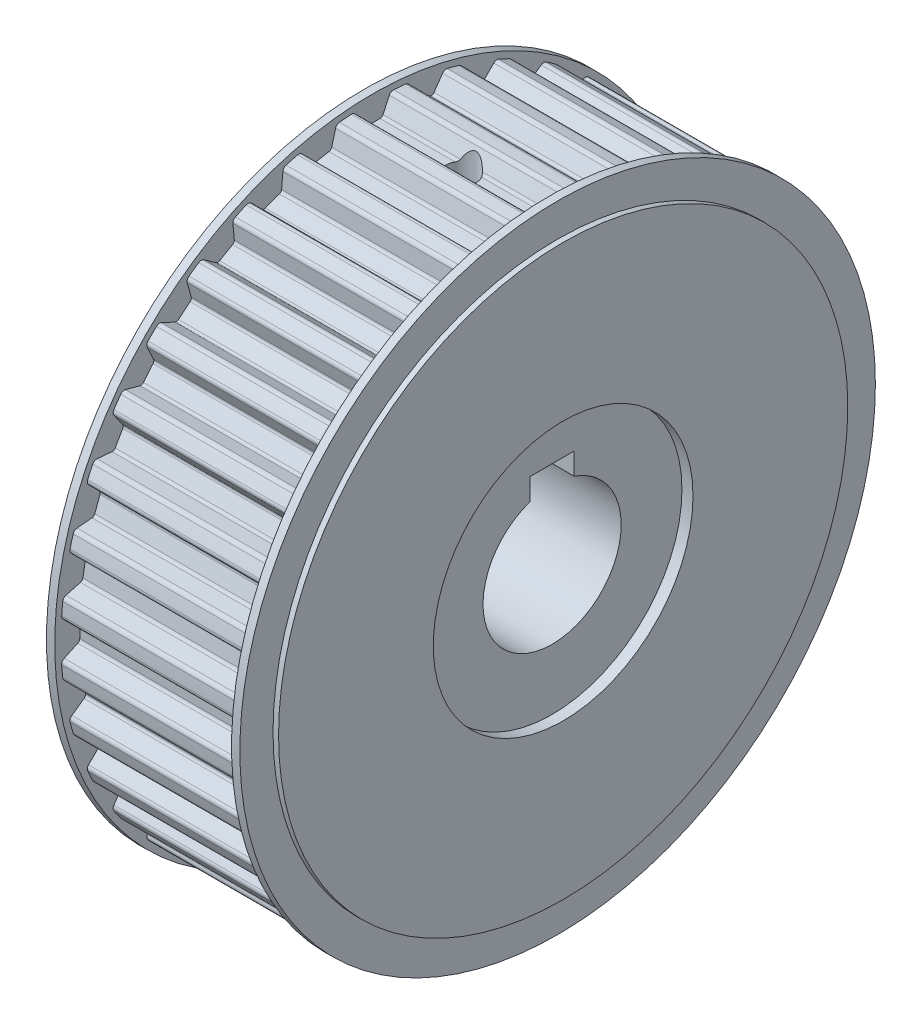
from build123d import *

# Parameters (mm, degrees)
SKETCH_1_R                       = 56.37
EXTRUDE_1_DEPTH                  = 16
CUT_EXTRUDE_2_DEPTH              = 32
FILLET_1_R                       = 0.6
FILLET_2_R                       = 0.8
PATTERN_CIRCULAR_1_COUNT         = 36
FILLET_1_OF_PATTERN_CIRCULAR_1_R = 0.6
FILLET_2_OF_PATTERN_CIRCULAR_1_R = 0.8
SKETCH_6_R                       = 57.5
EXTRUDE_2_DEPTH                  = 1.5
SKETCH_7_R                       = 51.5
EXTRUDE_3_DEPTH                  = 1
SKETCH_8_R                       = 12.5
CUT_EXTRUDE_1_DEPTH              = 90.339241098
SKETCH_11_W                      = 8
SKETCH_11_H                      = 9.02365329
CUT_EXTRUDE_3_DEPTH              = 25
HOLE_WIZARD_M4_1_D               = 3.3
HOLE_WIZARD_M4_1_DEPTH           = 47.1
HOLE_WIZARD_M4_1_TIP             = 0.991420021
SKETCH_14_R                      = 23.5
CUT_EXTRUDE_4_DEPTH              = 2
HOLE_WIZARD_5_5_5_5_1_D          = 5.5
HOLE_WIZARD_5_5_5_5_1_DEPTH      = 35
HOLE_WIZARD_5_5_5_5_1_TIP        = 1.652366702


with BuildPart() as part:
    # 草图1 → 拉伸1 (new, symmetric)
    with BuildSketch(Plane(origin=(0, 0, 0), x_dir=(0, 0, -1), z_dir=(1, 0, 0))):
        Circle(SKETCH_1_R)
    extrude(amount=EXTRUDE_1_DEPTH, both=True)

    # 草图2 → 拉伸2 (cut)
    with BuildSketch(Plane(origin=(16, 0, 0), x_dir=(0, 0, -1), z_dir=(1, 0, 0))):
        with BuildLine():
            Line((-3.285, 56.274200794), (-1.744225866, 52.97))
            Line((-1.744225866, 52.97), (1.744225866, 52.97))
            Line((1.744225866, 52.97), (3.285, 56.274200794))
            ThreePointArc((3.285, 56.274200794), (0, 56.37), (-3.285, 56.274200794))
        make_face()
    cut_extrude_2 = extrude(amount=-CUT_EXTRUDE_2_DEPTH, mode=Mode.SUBTRACT)

    # 圆角1
    fillet_1_edges = [part.edges().sort_by_distance(p)[0] for p in [
        (0, 52.97, -1.744225866),
        (0, 52.97, 1.744225866),
    ]]
    fillet(fillet_1_edges, radius=FILLET_1_R)

    # 圆角2
    fillet_2_edges = [part.edges().sort_by_distance(p)[0] for p in [
        (0, 56.274200794, 3.285),
        (0, 56.274200794, -3.285),
    ]]
    fillet(fillet_2_edges, radius=FILLET_2_R)

    # 阵列(圆周)1: 拉伸2 ×36 about axis
    pattern_circular_1_axis = Axis((0, 0, 0), (1, 0, 0))
    for i in range(1, PATTERN_CIRCULAR_1_COUNT):
        add(cut_extrude_2.rotate(pattern_circular_1_axis, i * 360 / PATTERN_CIRCULAR_1_COUNT), mode=Mode.SUBTRACT)

    # 圆角1 of 阵列(圆周)1
    fillet_1_of_pattern_circular_1_edges = [part.edges().sort_by_distance(p)[0] for p in [
        (0, 52.46814832, 7.480416815),
        (0, 51.862385034, 10.915871127),
        (0, 50.372078504, 16.477770817),
        (0, 49.178957742, 19.755843167),
        (0, 46.745478571, 24.97445609),
        (0, 45.001252706, 27.99554391),
        (0, 41.698540927, 32.712305153),
        (0, 39.456207377, 35.384614217),
        (0, 35.384614217, 39.456207377),
        (0, 32.712305153, 41.698540927),
        (0, 27.99554391, 45.001252706),
        (0, 24.97445609, 46.745478571),
        (0, 19.755843167, 49.178957742),
        (0, 16.477770817, 50.372078504),
        (0, 10.915871127, 51.862385034),
        (0, 7.480416815, 52.46814832),
        (0, 1.744225866, 52.97),
        (0, -1.744225866, 52.97),
        (0, -7.480416815, 52.46814832),
        (0, -10.915871127, 51.862385034),
        (0, -16.477770817, 50.372078504),
        (0, -19.755843167, 49.178957742),
        (0, -24.97445609, 46.745478571),
        (0, -27.99554391, 45.001252706),
        (0, -32.712305153, 41.698540927),
        (0, -35.384614217, 39.456207377),
        (0, -39.456207377, 35.384614217),
        (0, -41.698540927, 32.712305153),
        (0, -45.001252706, 27.99554391),
        (0, -46.745478571, 24.97445609),
        (0, -49.178957742, 19.755843167),
        (0, -50.372078504, 16.477770817),
        (0, -51.862385034, 10.915871127),
        (0, -52.46814832, 7.480416815),
        (0, -52.97, 1.744225866),
        (0, -52.97, -1.744225866),
        (0, -52.46814832, -7.480416815),
        (0, -51.862385034, -10.915871127),
        (0, -50.372078504, -16.477770817),
        (0, -49.178957742, -19.755843167),
        (0, -46.745478571, -24.97445609),
        (0, -45.001252706, -27.99554391),
        (0, -41.698540927, -32.712305153),
        (0, -39.456207377, -35.384614217),
        (0, -35.384614217, -39.456207377),
        (0, -32.712305153, -41.698540927),
        (0, -27.99554391, -45.001252706),
        (0, -24.97445609, -46.745478571),
        (0, -19.755843167, -49.178957742),
        (0, -16.477770817, -50.372078504),
        (0, -10.915871127, -51.862385034),
        (0, -7.480416815, -52.46814832),
        (0, -1.744225866, -52.97),
        (0, 1.744225866, -52.97),
        (0, 7.480416815, -52.46814832),
        (0, 10.915871127, -51.862385034),
        (0, 16.477770817, -50.372078504),
        (0, 19.755843167, -49.178957742),
        (0, 24.97445609, -46.745478571),
        (0, 27.99554391, -45.001252706),
        (0, 32.712305153, -41.698540927),
        (0, 35.384614217, -39.456207377),
        (0, 39.456207377, -35.384614217),
        (0, 41.698540927, -32.712305153),
        (0, 45.001252706, -27.99554391),
        (0, 46.745478571, -24.97445609),
        (0, 49.178957742, -19.755843167),
        (0, 50.372078504, -16.477770817),
        (0, 51.862385034, -10.915871127),
        (0, 52.46814832, -7.480416815),
    ]]
    fillet(fillet_1_of_pattern_circular_1_edges, radius=FILLET_1_OF_PATTERN_CIRCULAR_1_R)

    # 圆角2 of 阵列(圆周)1
    fillet_2_of_pattern_circular_1_edges = [part.edges().sort_by_distance(p)[0] for p in [
        (0, 54.848834973, 13.007005886),
        (0, 55.9897035, 6.536818949),
        (0, 51.756915056, 22.33380048),
        (0, 54.003987398, 16.160019962),
        (0, 47.092387465, 30.981993848),
        (0, 50.377387465, 25.292206946),
        (0, 40.996981511, 38.688815011),
        (0, 45.220096107, 33.65590302),
        (0, 33.65590302, 45.220096107),
        (0, 38.688815011, 40.996981511),
        (0, 25.292206946, 50.377387465),
        (0, 30.981993848, 47.092387465),
        (0, 16.160019962, 54.003987398),
        (0, 22.33380048, 51.756915056),
        (0, 6.536818949, 55.9897035),
        (0, 13.007005886, 54.848834973),
        (0, -3.285, 56.274200794),
        (0, 3.285, 56.274200794),
        (0, -13.007005886, 54.848834973),
        (0, -6.536818949, 55.9897035),
        (0, -22.33380048, 51.756915056),
        (0, -16.160019962, 54.003987398),
        (0, -30.981993848, 47.092387465),
        (0, -25.292206946, 50.377387465),
        (0, -38.688815011, 40.996981511),
        (0, -33.65590302, 45.220096107),
        (0, -45.220096107, 33.65590302),
        (0, -40.996981511, 38.688815011),
        (0, -50.377387465, 25.292206946),
        (0, -47.092387465, 30.981993848),
        (0, -54.003987398, 16.160019962),
        (0, -51.756915056, 22.33380048),
        (0, -55.9897035, 6.536818949),
        (0, -54.848834973, 13.007005886),
        (0, -56.274200794, -3.285),
        (0, -56.274200794, 3.285),
        (0, -54.848834973, -13.007005886),
        (0, -55.9897035, -6.536818949),
        (0, -51.756915056, -22.33380048),
        (0, -54.003987398, -16.160019962),
        (0, -47.092387465, -30.981993848),
        (0, -50.377387465, -25.292206946),
        (0, -40.996981511, -38.688815011),
        (0, -45.220096107, -33.65590302),
        (0, -33.65590302, -45.220096107),
        (0, -38.688815011, -40.996981511),
        (0, -25.292206946, -50.377387465),
        (0, -30.981993848, -47.092387465),
        (0, -16.160019962, -54.003987398),
        (0, -22.33380048, -51.756915056),
        (0, -6.536818949, -55.9897035),
        (0, -13.007005886, -54.848834973),
        (0, 3.285, -56.274200794),
        (0, -3.285, -56.274200794),
        (0, 13.007005886, -54.848834973),
        (0, 6.536818949, -55.9897035),
        (0, 22.33380048, -51.756915056),
        (0, 16.160019962, -54.003987398),
        (0, 30.981993848, -47.092387465),
        (0, 25.292206946, -50.377387465),
        (0, 38.688815011, -40.996981511),
        (0, 33.65590302, -45.220096107),
        (0, 45.220096107, -33.65590302),
        (0, 40.996981511, -38.688815011),
        (0, 50.377387465, -25.292206946),
        (0, 47.092387465, -30.981993848),
        (0, 54.003987398, -16.160019962),
        (0, 51.756915056, -22.33380048),
        (0, 55.9897035, -6.536818949),
        (0, 54.848834973, -13.007005886),
    ]]
    fillet(fillet_2_of_pattern_circular_1_edges, radius=FILLET_2_OF_PATTERN_CIRCULAR_1_R)

    # 草图6 → 凸台-拉伸2 (add)
    with BuildSketch(Plane(origin=(16, 0, 0), x_dir=(0, 0, -1), z_dir=(1, 0, 0))):
        Circle(SKETCH_6_R)
    extrude_2 = extrude(amount=EXTRUDE_2_DEPTH)

    # 草图7 → 凸台-拉伸3 (add)
    with BuildSketch(Plane(origin=(17.5, 0, 0), x_dir=(0, 0, -1), z_dir=(1, 0, 0))):
        Circle(SKETCH_7_R)
    extrude_3 = extrude(amount=EXTRUDE_3_DEPTH)

    # 镜向2: 凸台-拉伸2, 凸台-拉伸3 across plane
    add(extrude_2.mirror(Plane(origin=(0, 0, 0), x_dir=(0, 0, 1), z_dir=(1, 0, 0))))
    add(extrude_3.mirror(Plane(origin=(0, 0, 0), x_dir=(0, 0, 1), z_dir=(1, 0, 0))))

    # 草图8 → 切除-拉伸1 (cut, through all)
    with BuildSketch(Plane.ZY.offset(18.5)):
        Circle(SKETCH_8_R)
    extrude(amount=-CUT_EXTRUDE_1_DEPTH, mode=Mode.SUBTRACT)

    # 草图11 → 切除-拉伸3 (cut, symmetric)
    with BuildSketch(Plane(origin=(0, 0, 0), x_dir=(0, 0, -1), z_dir=(1, 0, 0))):
        with Locations((0, 11.288173355)):
            Rectangle(SKETCH_11_W, SKETCH_11_H)
    extrude(amount=CUT_EXTRUDE_3_DEPTH, both=True, mode=Mode.SUBTRACT)

    # M4 螺纹孔1
    with Locations(Plane(origin=(0, 56.37, 0), x_dir=(-1, 0, 0), z_dir=(0, 1, 0))):
        with Locations((0, 0)):
            Hole(HOLE_WIZARD_M4_1_D / 2, depth=HOLE_WIZARD_M4_1_DEPTH)
            with Locations((0, 0, -(HOLE_WIZARD_M4_1_DEPTH + HOLE_WIZARD_M4_1_TIP / 2))):  # 118° drill point
                Cone(0, HOLE_WIZARD_M4_1_D / 2, HOLE_WIZARD_M4_1_TIP, mode=Mode.SUBTRACT)

    # 草图14 → 切除-拉伸4 (cut)
    with BuildSketch(Plane(origin=(18.5, 0, 0), x_dir=(0, 0, -1), z_dir=(1, 0, 0))):
        Circle(SKETCH_14_R)
    cut_extrude_4 = extrude(amount=-CUT_EXTRUDE_4_DEPTH, mode=Mode.SUBTRACT)

    # 镜向3: 切除-拉伸4 across plane
    add(cut_extrude_4.mirror(Plane(origin=(0, 0, 0), x_dir=(0, 0, 1), z_dir=(1, 0, 0))), mode=Mode.SUBTRACT)

    # Ø5.5 (5.5) 直径孔1
    with Locations(Plane(origin=(0, 56.37, 0), x_dir=(1, 0, 0), z_dir=(0, 1, 0))):
        with Locations((0, 0)):
            Hole(HOLE_WIZARD_5_5_5_5_1_D / 2, depth=HOLE_WIZARD_5_5_5_5_1_DEPTH)
            with Locations((0, 0, -(HOLE_WIZARD_5_5_5_5_1_DEPTH + HOLE_WIZARD_5_5_5_5_1_TIP / 2))):  # 118° drill point
                Cone(0, HOLE_WIZARD_5_5_5_5_1_D / 2, HOLE_WIZARD_5_5_5_5_1_TIP, mode=Mode.SUBTRACT)


solid = part.part
